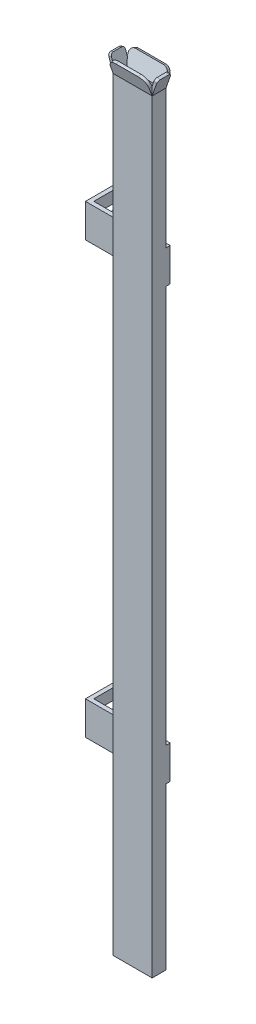
SolidWorks part; units mm, degrees
ref_plane "Front Plane" through (0, 0, 0) normal (0, 0, 1) x (1, 0, 0)
ref_plane "Top Plane" through (0, 0, 0) normal (0, 1, 0) x (1, 0, 0)
ref_plane "Right Plane" through (0, 0, 0) normal (1, 0, 0) x (0, 0, -1)
sketch "Sketch1" plane through (0, 0, 0) normal (0, 1, 0) x (1, 0, 0)
  line L1 (-6, 1.5) -> (6, 1.5)
  line L2 (-6, 1.5) -> (-6, -1.5)
  line L3 (-6, -1.5) -> (6, -1.5)
  line L4 (6, 1.5) -> (6, -1.5)
  line L5 (-6, 1.5) -> (6, -1.5) construction
  line L6 (-6, -1.5) -> (6, 1.5) construction
  line L7 (-7, 2.5) -> (7, 2.5)
  line L8 (-7, 2.5) -> (-7, -2.5)
  line L9 (-7, -2.5) -> (7, -2.5)
  line L10 (7, 2.5) -> (7, -2.5)
  line L11 (-7, 2.5) -> (7, -2.5) construction
  line L12 (-7, -2.5) -> (7, 2.5) construction
  point P0 (0, 0)
  point P6 (0, 0)
  dimension "D1" = 12
  dimension "D2" = 3
  dimension "D3" = 14
  dimension "D4" = 5
extrude "Boss-Extrude1" add sketch "Sketch1" along normal blind 275
sketch "Sketch2" plane through (0, 0, -2.5) normal (0, 0, -1) x (-1, 0, 0)
  line L0 (-7, 275) -> (-7, 0) construction
  line L1 (-7, 225) -> (22, 225)
  line L2 (-7, 225) -> (-7, 213)
  line L3 (-7, 213) -> (22, 213)
  line L4 (22, 225) -> (22, 213)
  line L5 (-7, 275) -> (7, 275) construction
  dimension "D1" = 12
  dimension "D2" = 29
  dimension "D3" = 50
extrude "Boss-Extrude2" add sketch "Sketch2" along normal blind 1.5
sketch "Sketch3" plane through (-22, 0, 0) normal (-1, 0, 0) x (0, 0, 1)
  line L1 (-2.5, 213) -> (-17.5, 213)
  line L2 (-2.5, 213) -> (-2.5, 225)
  line L3 (-2.5, 225) -> (-17.5, 225)
  line L4 (-17.5, 213) -> (-17.5, 225)
  dimension "D1" = 15
  dimension "D2" = 12
extrude "Boss-Extrude3" add sketch "Sketch3" against normal blind 1.5
pattern_linear "LPattern1" count 2 spacing 155 along (0, -1, 0) of "Boss-Extrude3", "Boss-Extrude2"
chamfer "Chamfer1" distance 1 angle 45 4 edges at (-21.25, 213, -17.5) (-21.25, 70, -17.5) (-21.25, 58, -17.5) (-21.25, 225, -17.5)
sketch "Sketch4" plane through (-20.5, 0, 0) normal (1, 0, 0) x (0, 0, -1)
  line L0 (17.5, 219) -> (-49982.5, 219) construction
  line L1 (17.5, 224) -> (17.5, 214) construction
  line L2 (17.5, 64) -> (-49982.5, 64) construction
  line L3 (17.5, 69) -> (17.5, 59) construction
  line L4 (4, 70) -> (4, 58) construction
  line L5 (8, 64) -> (14, 64) construction
  line L6 (8, 66) -> (14, 66)
  line L7 (8, 62) -> (14, 62)
  line L8 (14, 219) -> (8, 219) construction
  line L9 (14, 217.25) -> (8, 217.25)
  line L10 (14, 220.75) -> (8, 220.75)
  arc A0 (8, 66) -> (8, 62) centre (8, 64) ccw
  arc A1 (14, 62) -> (14, 66) centre (14, 64) ccw
  arc A2 (14, 217.25) -> (14, 220.75) centre (14, 219) ccw
  arc A3 (8, 220.75) -> (8, 217.25) centre (8, 219) ccw
  point P4 (17.5, 219)
  point P9 (17.5, 64)
  point P12 (4, 64)
  point P15 (11, 64)
  point P22 (11, 219)
  dimension "D1" = 4
  dimension "D2" = 3.5
  dimension "D3" = 3.5
  dimension "D4" = 6
extrude "Cut-Extrude1" cut sketch "Sketch4" against normal blind 10
sketch "Sketch5" plane through (7, 0, 0) normal (1, 0, 0) x (0, 0, -1)
  line L0 (-1.5, 275) -> (-3.5521, 280.6382)
  line L1 (-3.5521, 280.6382) -> (-4.4918, 280.2961)
  line L2 (-4.4918, 280.2961) -> (-1.5, 272.0762)
  line L3 (-1.5, 275) -> (-1.5, 0) construction
  line L4 (-2.5, 275) -> (-2.5, 0) construction
  line L6 (-1.5, 275) -> (-1.5, 272.0762)
  dimension "D1" = 1
  dimension "D2" = 160
  dimension "D3" = 6
extrude "Boss-Extrude4" add sketch "Sketch5" against normal up to surface (14 mm away) up to face at (-7, 139.5, -1.25)
fillet "Fillet1" radius 3 2 edges at (-7, 280.4671, 4.022) (7, 280.4671, 4.022)
sketch "Sketch6" plane through (0, 0, -2.5) normal (0, 0, -1) x (-1, 0, 0)
  line L0 (-6, 275) -> (-7.9534, 280.6731)
  line L1 (-7.9534, 280.6731) -> (-8.8989, 280.3475)
  line L2 (-8.8989, 280.3475) -> (-6, 271.9284)
  line L3 (-6, 275) -> (-6, 271.9284)
  line L5 (-6, 275) -> (-6, 0) construction
  line L6 (-6, 275) -> (-6, 0)
  line L7 (0, 280.6382) -> (0, -49719.3618) construction
  line L9 (4, 280.6382) -> (-4, 280.6382) construction
  line L10 (6, 275) -> (6, 271.9284)
  line L11 (8.8989, 280.3475) -> (6, 271.9284)
  line L12 (7.9534, 280.6731) -> (8.8989, 280.3475)
  line L13 (6, 275) -> (7.9534, 280.6731)
  point P13 (0, 280.6382)
  dimension "D1" = 1
  dimension "D2" = 6
  dimension "D3" = 38
extrude "Boss-Extrude5" add sketch "Sketch6" against normal up to surface (5 mm away) contours L0 L1 L2 L3 | L11 L10 L13 L12 up to face at (0, 137.4118, 2.5)
fillet "Fillet2" radius 1 4 edges at (-8.4262, 280.5103, 2.5) (-8.4262, 280.5103, -2.5) (8.4262, 280.5103, 2.5) (8.4262, 280.5103, -2.5)
ref_plane "Plane1" through (0, 0, 0) normal (0, 0, 1) x (1, 0, 0)
mirror "Mirror1" about plane through (0, 0, 0) normal (0, 0, 1) of "Boss-Extrude4"
fillet "Fillet3" radius 2 2 edges at (-7, 280.4671, -4.022) (7, 280.4671, -4.022)
